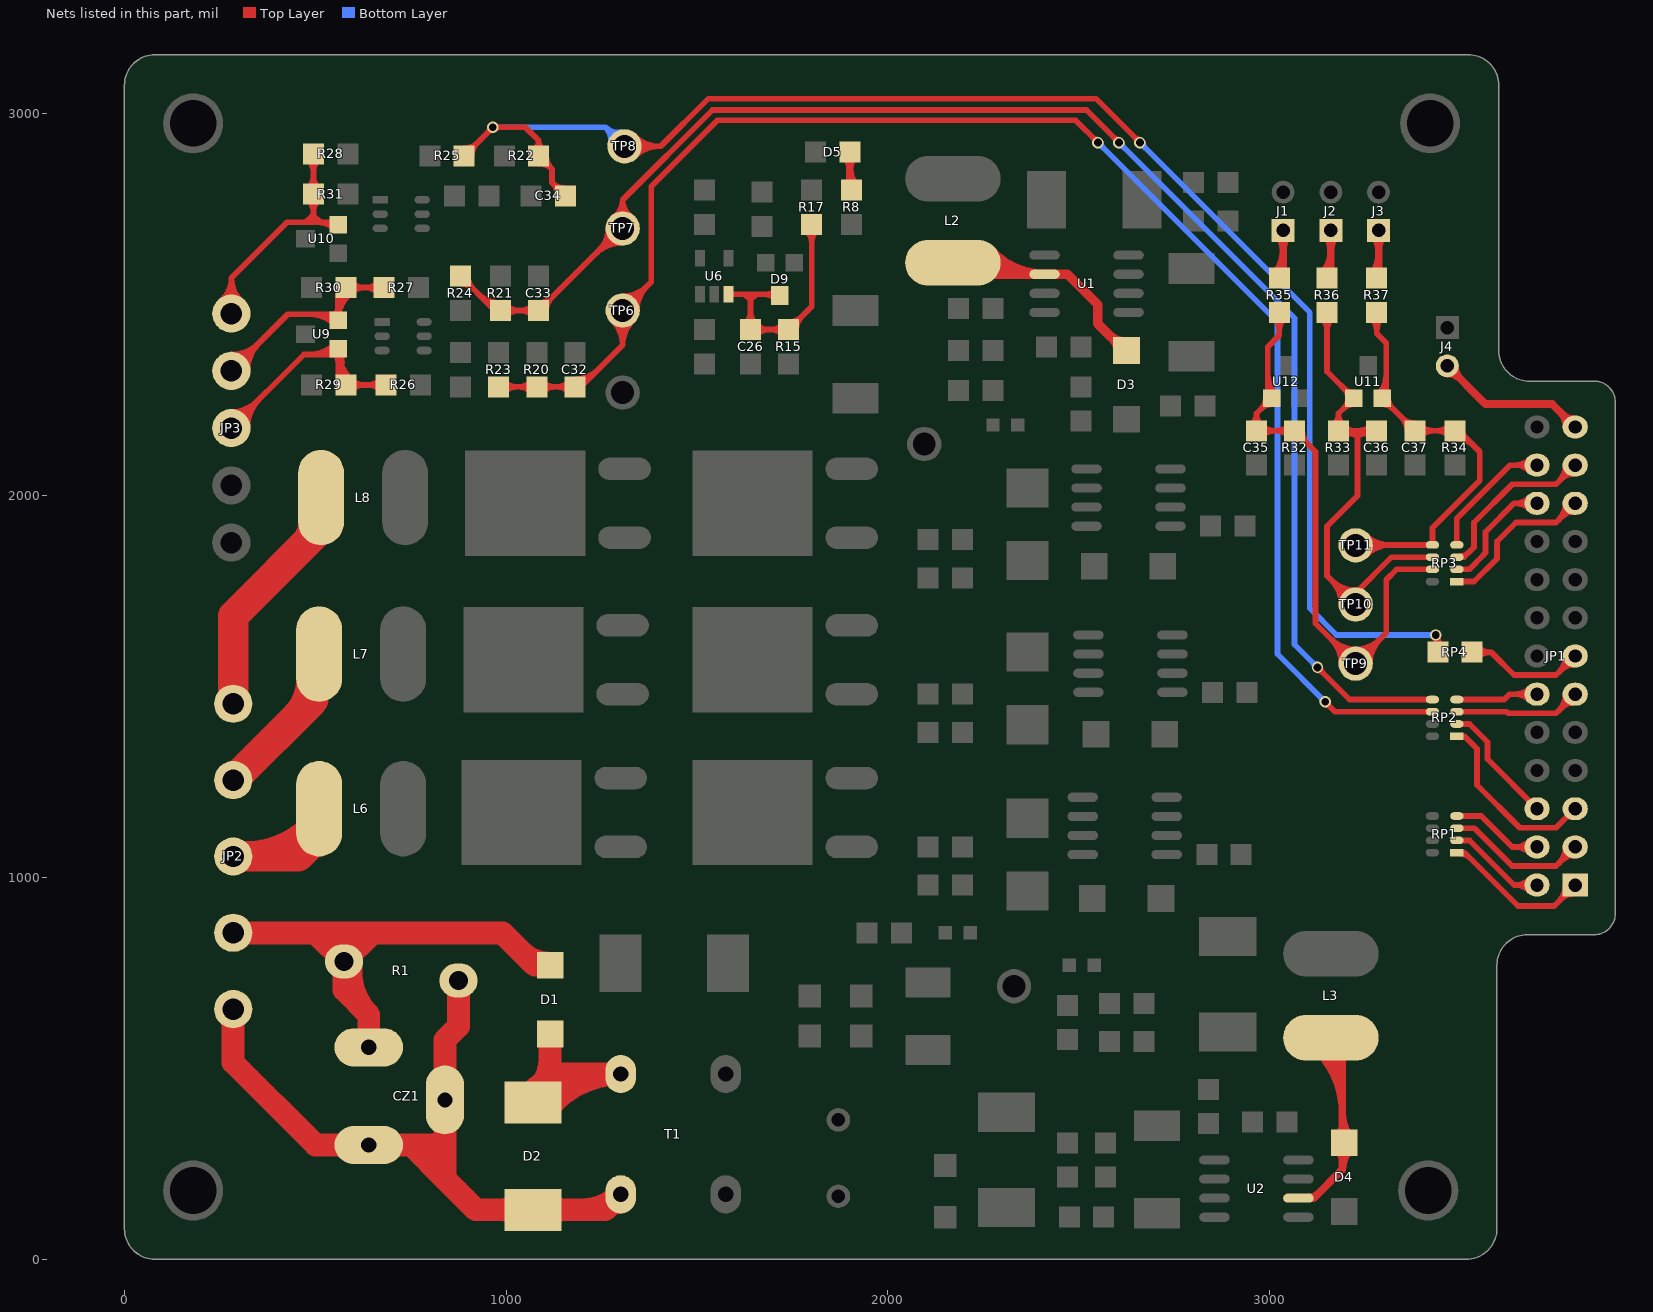
[diagram p0: the nets of this part, all layers, seen from the top]
# Altium PCB MISC103926.PcbDoc (part 3 of 4)
Units mil, origin at the board's own origin, x right, y up, seen from the top; angles counter-clockwise.
Board outline 3905 x 3155 mil, 4 copper layers (Top Layer, GND1, GND2, Bottom Layer); 132 components, 84 nets, 362 pads, 268 vias.

## Via types
v1: diameter 30, hole 20, Top Layer to Bottom Layer, 268 vias

## Nets (pads, with @x,y where several pads share a name; then routed paths per layer and width w, separated by ;. In a path a pad name is that pad's centre, name@x,y a point inside that pad or via, vN(x,y) a via of type N, cw(c..) or ccw(c..) an arc to the next point about the centre after c; other vN are vias at no path point) (continued)
NetC26_2: C26.2 D9.3 R15.1 R17.2 U6.3 | length 1114.7
  Top Layer w15: U6.3@1582.4,2527.76 1713.24,2527.76 D9.3@1717,2524 ; 1625,2527.76 1640,2512.76 ; C26.2@1625.86,2449.14 ccw(c1591.72,2483.28) 1640,2483.28 ccw(c1688.28,2483.28) 1654.14,2449.14 ccw(c1688.28,2483.28) 1688.28,2435 ccw(c1688.28,2386.72) C26.2@1654.14,2420.86 ; 1640,2527.76 1640,2510 ; 1655,2527.76 1640,2512.76 ; 1675.34,2527.76 cw(c1675.34,2484.34) D9.3@1706.04,2515.04 ; 1683.82,2527.76 ccw(c1683.82,2559.18) D9.3@1706.04,2536.96 ; R15.1@1725.86,2420.86 ccw(c1691.72,2386.72) 1691.72,2435 ccw(c1691.72,2483.28) R15.1@1725.86,2449.14 ; R15.1@1740,2455 ccw(c1740,2503.28) 1774.14,2469.14 ccw(c1808.28,2435) R15.1@1760,2435 ; R17.2@1785.86,2695.86 cw(c1751.72,2661.72) 1800,2661.72 cw(c1848.28,2661.72) R17.2@1814.14,2695.86 ; R17.2@1800,2710 1800,2495 R15.1@1740,2435 C26.2@1640,2435 1640,2510 ; 1640,2510 1640,2512.76 ; 1640,2510 1640,2512.76
NetC32_1: C32.1 R20.2 R23.1 RP2.6 TP6.1 | length 5058.5
  Top Layer w15: R23.1@985,2285 1195,2285 1305,2395 ; R23.1@994.14,2270.86 cw(c1028.28,2236.72) 1028.28,2285 cw(c1028.28,2333.28) R23.1@994.14,2299.14 ; R20.2@1065.86,2270.86 ccw(c1031.72,2236.72) 1031.72,2285 ccw(c1031.72,2333.28) R20.2@1065.86,2299.14 ; R20.2@1094.14,2270.86 cw(c1128.28,2236.72) 1128.28,2285 cw(c1128.28,2333.28) R20.2@1094.14,2299.14 ; C32.1@1165.86,2270.86 ccw(c1131.72,2236.72) 1131.72,2285 ccw(c1131.72,2333.28) C32.1@1165.86,2299.14 ; C32.1@1180,2290 ccw(c1180,2338.28) 1214.14,2304.14 ; C32.1@1180,2305 ccw(c1180,2389.5) 1239.75,2329.75 ; TP6.1@1278.6,2458.37 cw(c1215.76,2395.01) 1305,2395.01 ; TP6.1@1289.16,2469.02 cw(c1251.46,2431) 1305,2431 cw(c1358.54,2431) TP6.1@1320.84,2469.02 ; TP6.1@1305,2507.5 ccw(c1305,2561.82) 1343.41,2523.41 ccw(c1381.82,2485) TP6.1@1327.5,2485 ; TP6.1@1305,2522.5 ccw(c1305,2613.03) 1369.02,2549.02 ccw(c1433.03,2485) TP6.1@1342.5,2485 ; TP6.1@1331.4,2458.37 ccw(c1394.24,2395.01) 1305,2395.01 ; v1@2542.5,2925 ccw(c2524.39,2925) 2537.2,2937.8 ccw(c2550,2950.61) v1@2550,2932.5 ; v1(2550,2925) 2492,2983 1553,2983 1380,2810 1380,2560 TP6.1@1305,2485 1305,2395 ; v1@3145,1452.5 cw(c3145,1434.39) 3157.8,1447.2 cw(c3170.61,1460) v1@3152.5,1460 ; v1(3145,1460) 3171,1434 RP2.6@3426,1434
  Bottom Layer w15: v1@2550,2917.5 cw(c2550,2899.39) 2562.8,2912.2 cw(c2575.61,2925) v1@2557.5,2925 ; v1(2550,2925) 3020,2455 3020,1585 v1@3147.5,1457.5 ; v1@3137.5,1460 ccw(c3119.39,1460) 3132.2,1472.8 ccw(c3145,1485.61) v1@3145,1467.5
NetC33_1: C33.1 R21.2 R24.1 RP2.5 TP7.1 | length 4826.9
  Top Layer w15: R24.1@880,2555 cw(c880,2506.72) 914.14,2540.86 cw(c948.28,2575) R24.1@900,2575 ; R24.1@880,2575 R21.2@970,2485 ; 925.25,2529.75 ccw(c985,2589.5) R21.2@985,2505 ; 950.86,2504.14 ccw(c985,2538.28) R21.2@985,2490 ; R21.2@985,2485 C33.1@1090,2485 ; R21.2@999.14,2470.86 cw(c1033.28,2436.72) 1033.28,2485 cw(c1033.28,2533.28) R21.2@999.14,2499.14 ; C33.1@1070.86,2470.86 ccw(c1036.72,2436.72) 1036.72,2485 ccw(c1036.72,2533.28) C33.1@1070.86,2499.14 ; C33.1@1085,2485 TP7.1@1302.5,2702.5 ; C33.1@1085,2505 ccw(c1085,2553.28) 1119.14,2519.14 ccw(c1153.28,2485) C33.1@1105,2485 ; 1232.45,2632.45 cw(c1305,2559.9) TP7.1@1305,2662.5 ; 1244.52,2644.52 ccw(c1189.04,2700) TP7.1@1267.5,2700 ; 1258.05,2658.05 cw(c1305,2611.11) TP7.1@1305,2677.5 ; 1270.13,2670.13 ccw(c1240.25,2700) TP7.1@1282.5,2700 ; TP7.1@1282.5,2730 ccw(c1248.76,2775) 1305,2775 ; TP7.1@1305,2700 1305,2775 ; TP7.1@1327.5,2730 cw(c1361.24,2775) 1305,2775 ; v1@2597.5,2925 ccw(c2579.39,2925) 2592.2,2937.8 ccw(c2605,2950.61) v1@2605,2932.5 ; v1(2605,2925) 2520,3010 1540,3010 1305,2775 ; v1@3125,1542.5 cw(c3125,1524.39) 3137.8,1537.2 cw(c3150.61,1550) v1@3132.5,1550 ; v1(3125,1550) 3209,1466 RP2.5@3426,1466
  Bottom Layer w15: v1@2605,2917.5 cw(c2605,2899.39) 2617.8,2912.2 cw(c2630.61,2925) v1@2612.5,2925 ; v1(2605,2925) 3065,2465 3065,1610 v1(3125,1550) ; v1@3117.5,1550 ccw(c3099.39,1550) 3112.2,1562.8 ccw(c3125,1575.61) v1@3125,1557.5
NetC34_1: C34.1 R22.2 R25.1 RP4.2 TP8.1 | length 4924.8
  Top Layer w15: R25.1@890,2890 v1(965,2965) 1050,2965 1085,2930 ; R25.1@890,2910 ccw(c890,2958.28) 924.14,2924.14 ccw(c958.28,2890) R25.1@910,2890 ; v1@957.5,2965 cw(c939.4,2965) 952.2,2952.2 cw(c965,2939.4) v1@965,2957.5 ; v1@970.31,2959.7 cw(c983.1,2946.91) 983.1,2965 cw(c983.12,2983.12) v1@970.31,2970.31 ; R22.2@1073,2906 ccw(c1055,2930) 1085,2930 ; R22.2@1085,2870 cw(c1085,2821.72) 1119.14,2855.86 cw(c1153.28,2890) R22.2@1105,2890 ; R22.2@1097,2906 cw(c1115,2930) 1085,2930 ; C34.1@1135,2785 ccw(c1086.72,2785) 1120.86,2819.14 ccw(c1155,2853.28) C34.1@1155,2805 ; C34.1@1150,2790 1120,2820 1120,2855 R22.2@1085,2890 1085,2930 ; TP8.1@1310,2915 1405,2915 1530,3040 2545,3040 v1(2660,2925) ; TP8.1@1325.91,2899.09 cw(c1364.32,2860.68) 1364.32,2915 cw(c1364.32,2969.32) TP8.1@1325.91,2930.91 ; TP8.1@1336.52,2888.48 cw(c1400.53,2824.47) 1400.53,2915 cw(c1400.53,3005.53) TP8.1@1336.52,2941.52 ; v1@2652.5,2925 ccw(c2634.39,2925) 2647.2,2937.8 ccw(c2660,2950.61) v1@2660,2932.5 ; v1@2657.5,2922.5 v1@2657.5,2932.5 ; RP4.2@3428,1606 ccw(c3410,1630) v1@3440,1630 ; v1@3429.7,1629.7 cw(c3404.82,1604.82) RP4.2@3440,1604.82 ; v1@3431.25,1628.5 cw(c3416.16,1602.37) RP4.2@3445.31,1610.18 ; v1(3435,1635) v1@3440,1630 ; RP4.2@3440,1590 v1@3440,1630 ; RP4.2@3452,1606 cw(c3470,1630) v1@3440,1630
  Bottom Layer w15: v1(965,2965) 1260,2965 ; v1@970.31,2959.7 cw(c983.1,2946.91) 983.1,2965 cw(c983.12,2983.12) v1@970.31,2970.31 ; TP8.1@1273.17,2922.08 ccw(c1226.12,2931.12) 1260,2965 ; TP8.1@1302.92,2951.83 cw(c1293.88,2998.88) 1260,2965 ; TP8.1@1310,2915 1260,2965 ; v1@2660,2917.5 cw(c2660,2899.39) 2672.8,2912.2 cw(c2685.61,2925) v1@2667.5,2925 ; v1(2660,2925) 3105,2480 3105,1705 3175,1635 v1(3435,1635) ; v1@3429.7,1629.7 ccw(c3416.89,1616.89) 3416.89,1635 ccw(c3416.89,1653.11) v1@3429.7,1640.3
NetC35_2: C35.2 R32.1 R35.2 RP3.7 TP9.1 U12.1 | length 2488.9
  Top Layer w15: C35.2@2951.6,2184.85 ccw(c2924.38,2215) 2965,2215 ; C35.2@2978.4,2184.85 cw(c3005.62,2215) 2965,2215 ; C35.2@2979.14,2155.86 cw(c3013.28,2121.72) 3013.28,2170 cw(c3013.28,2218.28) C35.2@2979.14,2184.14 ; U12.1@2989.5,2255 cw(c2952.08,2255) 2978.54,2228.54 cw(c3005,2202.08) U12.1@3005,2239.5 ; 2995,2280.35 ccw(c3030.35,2280.35) U12.1@3005.35,2255.35 ; 2995,2316.56 ccw(c3066.56,2316.56) U12.1@3015.96,2265.96 ; R35.2@3010.86,2465.86 cw(c2976.72,2431.72) 3025,2431.72 cw(c3073.28,2431.72) R35.2@3039.14,2465.86 ; R35.2@3025,2470 R35.2@3025,2480 3025,2420 2995,2390 2995,2265 U12.1@3005,2255 2965,2215 ; R32.1@3050.86,2155.86 ccw(c3016.72,2121.72) 3016.72,2170 ccw(c3016.72,2218.28) R32.1@3050.86,2184.14 ; R32.1@3065,2150 cw(c3065,2101.72) 3099.14,2135.86 cw(c3133.28,2170) R32.1@3085,2170 ; R32.1@3065,2170 3120,2115 3120,1665 TP9.1@3225,1560 3305,1640 3305,1780 3332,1807 RP3.7@3426,1807 ; R32.1@3070,2170 C35.2@2965,2170 2965,2215 ; TP9.1@3187.5,1560 ccw(c3096.97,1560) 3160.98,1624.02 ccw(c3225,1688.03) 3225,1597.5 ccw(c3225,1688.03) 3289.02,1624.02 ccw(c3353.03,1560) TP9.1@3262.5,1560 ; TP9.1@3202.5,1560 ccw(c3148.18,1560) 3186.59,1598.41 ccw(c3225,1636.82) 3225,1582.5 ccw(c3225,1636.82) 3263.41,1598.41 ccw(c3301.82,1560) TP9.1@3247.5,1560
NetC36_2: C36.2 R33.1 R36.2 RP3.6 TP10.1 U11.1 | length 2143.9
  Top Layer w15: R36.2@3135.86,2465.86 cw(c3101.72,2431.72) 3150,2431.72 cw(c3198.28,2431.72) R36.2@3164.14,2465.86 ; R36.2@3150,2480 3150,2325 U11.1@3220,2255 3180,2215 ; R33.1@3166.6,2184.85 ccw(c3139.38,2215) 3180,2215 ; R33.1@3183.44,2166.37 cw(c3201.03,2147.82) 3219.11,2165.89 ; TP10.1@3187.5,1715 ccw(c3096.97,1715) 3160.98,1779.02 ccw(c3225,1843.03) TP10.1@3225,1752.5 ; R33.1@3193.4,2184.85 cw(c3220.62,2215) 3180,2215 ; R33.1@3193.76,2155.49 cw(c3211.63,2136.63) 3230,2155 ; R33.1@3196,2158 cw(c3220,2140) 3220,2170 ; R33.1@3196,2182 ccw(c3220,2200) 3220,2170 ; R33.1@3197.23,2159.85 cw(c3215,2149.38) 3215,2170 ; R33.1@3197.23,2180.15 ccw(c3215,2190.62) 3215,2170 ; R33.1@3198.46,2162.31 cw(c3210,2157.5) 3210,2170 ; R33.1@3198.46,2177.69 ccw(c3210,2182.5) 3210,2170 ; TP10.1@3202.5,1715 ccw(c3148.18,1715) 3186.59,1753.41 ccw(c3225,1791.82) TP10.1@3225,1737.5 ; U11.1@3220,2239.5 ccw(c3220,2202.08) 3193.54,2228.54 ccw(c3167.08,2255) 3204.5,2255 ccw(c3167.08,2255) 3193.54,2281.46 ccw(c3220,2307.92) U11.1@3220,2270.5 ; 3230,2170 3230,2155 ; 3240.89,2165.89 cw(c3258.97,2147.82) C36.2@3276.56,2166.37 ; 3245,2170 3230,2155 ; C36.2@3265.86,2155.86 ccw(c3231.72,2121.72) 3231.72,2170 ccw(c3231.72,2218.28) C36.2@3265.86,2184.14 ; C36.2@3266.24,2155.49 ccw(c3248.37,2136.63) 3230,2155 ; C36.2@3280,2170 3220,2170 ; RP3.6@3426,1839 3319,1839 3225,1745 TP10.1@3225,1715 3150,1790 3150,1920 3230,2000 3230,2155 ; 3180,2215 R33.1@3180,2170 3220,2170 ; 3210,2170 3215,2170 ; 3215,2170 3230,2155
NetC37_2: C37.2 R34.1 R37.2 RP3.5 TP11.1 U11.2 | length 1835.7
  Top Layer w15: TP11.1@3225,1870 3226,1871 RP3.5@3426,1871 3426,1916 3550,2040 3550,2115 3495,2170 R34.1@3485,2170 C37.2@3380,2170 U11.2@3295,2255 3305,2265 3305,2400 3280,2425 R37.2@3280,2480 R37.2@3286,2474 ; TP11.1@3240.91,1854.09 cw(c3281.74,1813.26) 3281.74,1871 ; TP11.1@3240.91,1885.91 ccw(c3276.9,1921.9) 3276.9,1871 ; TP11.1@3251.52,1843.48 cw(c3317.95,1777.05) 3317.95,1871 ; TP11.1@3251.52,1896.52 ccw(c3313.12,1958.12) 3313.12,1871 ; R37.2@3265.86,2465.86 cw(c3231.72,2431.72) 3280,2431.72 cw(c3328.28,2431.72) R37.2@3294.14,2465.86 ; U11.2@3284.04,2265.96 ccw(c3233.43,2316.56) 3305,2316.56 ; U11.2@3294.65,2255.35 ccw(c3269.65,2280.35) 3305,2280.35 ; U11.2@3295,2239.5 cw(c3295,2202.08) 3321.46,2228.54 cw(c3347.92,2255) U11.2@3310.5,2255 ; C37.2@3360,2170 ccw(c3311.72,2170) 3345.86,2204.14 ccw(c3380,2238.28) C37.2@3380,2190 ; C37.2@3394.14,2155.86 cw(c3428.28,2121.72) 3428.28,2170 cw(c3428.28,2218.28) C37.2@3394.14,2184.14 ; R34.1@3470.86,2155.86 ccw(c3436.72,2121.72) 3436.72,2170 ccw(c3436.72,2218.28) R34.1@3470.86,2184.14 ; R34.1@3485,2150 cw(c3485,2077.57) 3536.21,2128.79 ; R34.1@3485,2165 cw(c3485,2128.79) R34.1@3510.61,2154.39 ; R34.1@3505,2170 ccw(c3529.14,2170) R34.1@3512.07,2152.93
NetCZ1_1: CZ1.1 CZ1.3 D2.2 JP2.1 R1.2 T1.1 | length 2284.5
  Top Layer w60: JP2.1@284.55,654.55 284.55,515.45 500.91,299.09 833.46,299.09 839.37,305 ; 750.91,299.09 839.37,210.63 ; R1.2@875,730 875,610 839.37,574.37 CZ1.1@839.37,417.2 839.37,210.63 ; D2.2@1032.32,111.82 ccw(c989.64,69.14) 989.64,129.5 ccw(c989.64,189.86) D2.2@1032.32,147.18 ; D2.2@1107.68,111.82 cw(c1150.36,69.14) 1150.36,129.5 cw(c1150.36,189.86) D2.2@1107.68,147.18 ; 1202.22,129.5 ccw(c1202.22,257.78) T1.1@1292.93,167.07 ; 1265.86,135.86 cw(c1300,101.72) T1.1@1300,150 ; T1.1@1300,170 1259.5,129.5 D2.2@1070,129.5 920.5,129.5 839.37,210.63
NetCZ1_2: CZ1.2 D1.2 JP2.2 R1.1 | length 1572
  Top Layer w60: JP2.2@285,855 500,855 ; R1.1@570,775 R1.1@575,780 ; R1.1@594.83,777.73 ccw(c753.48,753.49) 640,640 ; CZ1.2@640,555 640,640 ; 1038.18,806.82 ccw(c1115,883.64) D1.2@1115,775 ; D1.2@1115,770 1075,770 990,855 650,855 ; 500,855 R1.1@575,780 ; 500,855 650,855 ; R1.1@575,780 575,705 640,640 ; R1.1@575,780 650,855
NetD1_1: D1.1 D2.1 T1.4 | length 841.9
  Top Layer w60: D2.1@1062.91,432.67 cw(c1173.36,342.28) 1173.36,485 ; D2.1@1070,410.5 1115,455.5 D1.1@1115,590 ; D2.1@1072.32,428.18 ccw(c969.29,531.21) 1115,531.21 ; D2.1@1109.35,394.67 cw(c1299.99,238.66) T1.4@1300,485 1115,485
NetD3_1: D3.1 L2.1 U1.2 | length 1009
  Top Layer w25: L2.1@2170,2610 2200,2580 U1.2@2410,2580 ; L2.1@2233.15,2608.32 ccw(c2297.09,2666.35) 2297.09,2580 ; L2.1@2251.66,2625.12 ccw(c2353.54,2717.58) 2353.54,2580 ; L2.1@2270.18,2641.92 ccw(c2409.99,2768.8) U1.2@2410,2580 ; 2578.05,2421.95 ccw(c2625,2468.89) D3.1@2625,2402.5 ; D3.1@2590.13,2409.87 cw(c2560.25,2380) D3.1@2602.5,2380 ; D3.1@2625,2380 2620,2380 2550,2450 2550,2500 2470,2580 U1.2@2410,2580
NetD4_1: D4.1 L3.1 U2.2 | length 1143.2
  Top Layer w20: U2.2@3075,160 3115,160 3190,235 3190,305 3190,550 L3.1@3160,580 L3.1@3150,570 ; U2.2@3103,162 ccw(c3103,195.8) 3126.9,171.9 ; L3.1@3124.65,544.64 cw(c2966.87,386.86) 3190,386.86 ; L3.1@3138.79,558.79 cw(c3015.15,435.15) 3190,435.15 ; L3.1@3152.93,572.93 cw(c3063.43,483.43) 3190,483.43 ; D4.1@3177.32,287.32 cw(c3146.72,256.72) 3190,256.72 ; D4.1@3177.32,322.68 ccw(c3146.72,353.28) 3190,353.28 ; 3190,234.83 cw(c3262.07,234.83) D4.1@3212.27,286.93 ; 3190,377.43 ccw(c3267.43,377.43) D4.1@3212.68,322.68
NetD5_1: D5.1 R8.2 | length 234.8
  Top Layer w20: D5.1@1887.63,2887.63 cw(c1857.75,2857.75) 1900,2857.75 cw(c1942.25,2857.75) D5.1@1912.37,2887.63 ; R8.2@1892.63,2812.37 ccw(c1874.82,2830.18) 1900,2830.18 ; 1900,2854.32 ccw(c1959.32,2854.32) R8.2@1917.37,2812.37 ; D5.1@1900,2900 1900,2805 R8.2@1905,2800
NetJ1_1: J1.1 R35.1 | length 265
  Top Layer w15: R35.1@3025,2570 R35.1@3035,2580
  Top Layer w20: R35.1@3012.63,2582.37 ccw(c2958.61,2636.39) 3035,2636.39 ; J1.1@3020.86,2680.86 cw(c2986.72,2646.72) 3035,2646.72 cw(c3083.29,2646.72) J1.1@3049.14,2680.86 ; R35.1@3035,2580 J1.1@3035,2695
NetJ2_1: J2.1 R36.1 | length 265
  Top Layer w15: R36.1@3150,2570 R36.1@3160,2580
  Top Layer w20: R36.1@3137.63,2582.37 ccw(c3083.61,2636.39) 3160,2636.39 ; J2.1@3145.86,2680.86 cw(c3111.72,2646.72) 3160,2646.72 cw(c3208.29,2646.72) J2.1@3174.14,2680.86 ; R36.1@3160,2580 J2.1@3160,2695
NetJ3_1: J3.1 R37.1 | length 269.3
  Top Layer w15: R37.1@3280,2570 R37.1@3285,2575
  Top Layer w20: R37.1@3267.63,2582.37 ccw(c3225.68,2624.32) 3285,2624.32 ; J3.1@3270.86,2680.86 cw(c3236.72,2646.72) 3285,2646.72 cw(c3333.29,2646.72) J3.1@3299.14,2680.86 ; R37.1@3285,2575 J3.1@3285,2695 ; 3285,2600.18 ccw(c3310.18,2600.18) R37.1@3292.37,2582.37
NetJ4_2: J4.2 JP1.25 | length 553
  Top Layer w20: J4.2@3465,2320 cw(c3465,2271.72) 3499.14,2305.86 cw(c3533.28,2340) J4.2@3485,2340 ; J4.2@3465,2340 3565,2240 3740,2240 JP1.25@3800,2180 ; 3760.74,2219.26 cw(c3721.47,2180) JP1.25@3777,2180 ; 3767.98,2212.02 ccw(c3797,2241.04) JP1.25@3797,2200
NetJP1_1: JP1.1 RP1.1 | length 504.5
  Top Layer w15: RP1.1@3490,1065 3510,1065 3650,925 3745,925 JP1.1@3800,980 ; RP1.1@3497.5,1062.5 cw(c3497.5,1026.29) 3523.11,1051.89 ; 3756.47,936.47 ccw(c3712.94,980) JP1.1@3774.5,980 ; 3763.71,943.71 cw(c3797,910.42) JP1.1@3797,957.5
NetJP1_2: JP1.2 RP1.2 | length 343.8
  Top Layer w15: RP1.2@3490,1097 3523,1097 3640,980 JP1.2@3700,980 ; JP1.2@3681.09,964.09 ccw(c3642.68,925.68) 3642.68,980 ccw(c3642.68,1034.32) JP1.2@3681.09,995.91
NetJP1_3: JP1.3 RP1.3 | length 457
  Top Layer w15: RP1.3@3490,1129 3536,1129 3635,1030 3750,1030 JP1.3@3800,1080 ; 3756.47,1036.47 ccw(c3712.94,1080) JP1.3@3774.5,1080 ; 3763.71,1043.71 cw(c3797,1010.42) JP1.3@3797,1057.5
NetJP1_4: JP1.4 RP1.4 | length 328.9
  Top Layer w15: RP1.4@3490,1161 3554,1161 3635,1080 JP1.4@3700,1080 ; JP1.4@3681.09,1064.09 ccw(c3642.68,1025.68) 3642.68,1080 ccw(c3642.68,1134.32) JP1.4@3681.09,1095.91
NetJP1_5: JP1.5 RP2.1 | length 485.8
  Top Layer w15: RP2.1@3490,1370 3510,1370 3543,1337 3543,1242 3655,1130 3750,1130 JP1.5@3800,1180
NetJP1_6: JP1.6 RP2.2 | length 328.3
  Top Layer w15: RP2.2@3490,1402 3523,1402 3570,1355 3570,1310 JP1.6@3700,1180
NetJP1_11: JP1.11 RP2.3 | length 417.7
  Top Layer w15: RP2.3@3490,1434 3620,1434 3624,1430 3750,1430 JP1.11@3800,1480 ; 3756.47,1436.47 ccw(c3712.94,1480) JP1.11@3774.5,1480 ; 3763.71,1443.71 cw(c3797,1410.42) JP1.11@3797,1457.5
NetJP1_12: JP1.12 RP2.4 | length 301.1
  Top Layer w15: RP2.4@3490,1466 3614,1466 3628,1480 JP1.12@3700,1480 ; JP1.12@3681.09,1464.09 ccw(c3642.68,1425.68) 3642.68,1480 ccw(c3642.68,1534.32) JP1.12@3681.09,1495.91
NetJP1_13: JP1.13 RP4.1 | length 476.7
  Top Layer w15: RP4.1@3530,1590 3580,1590 3640,1530 3750,1530 JP1.13@3800,1580 ; RP4.1@3544.14,1575.86 cw(c3578.28,1541.72) 3578.28,1590 cw(c3578.28,1638.28) RP4.1@3544.14,1604.14 ; 3756.47,1536.47 ccw(c3712.94,1580) JP1.13@3774.5,1580 ; 3763.71,1543.71 cw(c3797,1510.42) JP1.13@3797,1557.5
NetJP1_21: JP1.21 RP3.1 | length 506.6
  Top Layer w15: RP3.1@3490,1775 3535,1775 3595,1835 3595,1880 3645,1930 3750,1930 JP1.21@3800,1980 ; 3756.47,1936.47 ccw(c3712.94,1980) JP1.21@3774.5,1980 ; 3763.71,1943.71 cw(c3797,1910.42) JP1.21@3797,1957.5
NetJP1_22: JP1.22 RP3.2 | length 399.4
  Top Layer w15: RP3.2@3490,1807 3522.36,1807 3560,1844.64 3560,1845 3565.18,1850.18 3565.18,1905.18 3640,1980 JP1.22@3700,1980 ; JP1.22@3681.09,1964.09 ccw(c3642.68,1925.68) 3642.68,1980 ccw(c3642.68,2034.32) JP1.22@3681.09,1995.91
NetJP1_23: JP1.23 RP3.3 | length 559.8
  Top Layer w15: RP3.3@3490,1839 3509,1839 3535,1865 3535,1930 3635,2030 3750,2030 JP1.23@3800,2080 ; RP3.3@3497.5,1841.5 ccw(c3497.5,1875.3) 3521.4,1851.4 ; 3756.47,2036.47 ccw(c3712.94,2080) JP1.23@3774.5,2080 ; 3763.71,2043.71 cw(c3797,2010.42) JP1.23@3797,2057.5
NetJP1_24: JP1.24 RP3.4 | length 422.3
  Top Layer w15: RP3.4@3490,1871 3490,1940 3630,2080 JP1.24@3700,2080 ; JP1.24@3681.09,2064.09 ccw(c3642.68,2025.68) 3642.68,2080 ccw(c3642.68,2134.32) JP1.24@3681.09,2095.91
NetJP2_3: JP2.3 L6.2 | length 510.4
  Top Layer w60: L6.2@495,1095 L6.2@495,1180
  Top Layer w80: JP2.3@285,1055 455,1055 L6.2@495,1095 ; JP2.3@316.86,1055 ccw(c316.86,1308.14) L6.2@495.86,1129.14
NetJP2_4: JP2.4 L7.2 | length 566.1
  Top Layer w60: L7.2@485,1585 L7.2@510,1560
  Top Layer w80: JP2.4@285,1255 495,1465 L7.2@495,1585 ; 447.57,1417.57 ccw(c345.14,1520) L7.2@490,1520
NetJP2_5: JP2.5 L8.2 | length 701.6
  Top Layer w80: JP2.5@285,1455 285,1685 515,1915 L8.2@515,1995 ; 470.25,1870.25 ccw(c410.5,1930) L8.2@495,1930
NetJP3_3: JP3.3 R26.2 R29.1 U9.1 | length 1401.1
  Top Layer w15: JP3.3@278.5,2178.5 470,2370 U9.1@560,2370 ; JP3.3@280,2204.5 ccw(c280,2263.65) 321.82,2221.82 ; JP3.3@280,2219.5 ccw(c280,2314.86) 347.43,2247.43 ; JP3.3@307.5,2177 cw(c381.13,2177) 329.07,2229.07 ; JP3.3@322.5,2177 cw(c432.35,2177) 354.67,2254.67 ; 486.37,2370 ccw(c486.37,2458.63) U9.1@549.04,2395.96 ; 522.58,2370 ccw(c522.58,2422.42) U9.1@559.65,2385.35 ; U9.1@549.04,2374.04 cw(c522.58,2347.58) 560,2347.58 cw(c597.42,2347.58) U9.1@570.96,2374.04 ; U9.1@552.25,2371.58 cw(c533.54,2339.17) 569.68,2348.86 cw(c605.83,2358.54) U9.1@573.42,2377.25 ; R29.1@560,2313.75 ccw(c603.2,2313.75) R29.1@573.01,2282.85 ; 560,2349.37 ccw(c638,2349.37) R29.1@583.49,2293.58 ; R29.1@593.98,2304.31 cw(c672.8,2384.99) U9.1@560,2385 560,2310 R29.1@580,2290 R26.2@685,2290 ; R29.1@594.14,2275.86 cw(c628.28,2241.72) 628.28,2290 cw(c628.28,2338.28) R29.1@594.14,2304.14 ; R26.2@670.86,2275.86 ccw(c636.72,2241.72) 636.72,2290 ccw(c636.72,2338.28) R26.2@670.86,2304.14
NetJP3_4: JP3.4 R27.2 R30.1 U9.2 | length 1296.2
  Top Layer w15: JP3.4@280,2327 428,2475 U9.2@559,2475 ; JP3.4@280,2354.5 ccw(c280,2420.89) 326.95,2373.95 ccw(c373.89,2327) JP3.4@307.5,2327 ; JP3.4@280,2369.5 ccw(c280,2472.1) 352.55,2399.55 ccw(c425.1,2327) JP3.4@322.5,2327 ; 486.36,2475 cw(c486.36,2386.36) U9.2@549.04,2449.04 ; 522.58,2475 cw(c522.58,2422.58) U9.2@559.65,2459.65 ; U9.2@549.04,2470.96 ccw(c524.99,2495.01) 559,2495.01 ; U9.2@559,2458.42 cw(c650.92,2458.42) R30.1@592.67,2529.53 ; 559,2490.09 cw(c624.97,2490.09) R30.1@583.17,2541.13 ; 559,2499.83 ccw(c599.83,2499.83) U9.2@570.96,2470.96 ; R30.1@559,2521.77 cw(c599.03,2521.77) R30.1@573.66,2552.74 ; U9.2@560,2460 559,2461 559,2524 R30.1@580,2545 R27.2@680,2545 ; R30.1@594.14,2530.86 cw(c628.28,2496.72) 628.28,2545 cw(c628.28,2593.28) R30.1@594.14,2559.14 ; R27.2@665.86,2530.86 ccw(c631.72,2496.72) 631.72,2545 ccw(c631.72,2593.28) R27.2@665.86,2559.14
NetJP3_5: JP3.5 R28.2 R31.1 U10.2 | length 1185.3
  Top Layer w15: JP3.5@252.19,2509.13 ccw(c199.51,2570) 280,2570 ; JP3.5@262,2497.79 ccw(c227.92,2537.17) 280,2537.17 ccw(c332.08,2537.17) JP3.5@298,2497.79 ; JP3.5@280,2477 280,2570 ; JP3.5@307.81,2509.13 cw(c360.49,2570) 280,2570 ; 475,2716 494,2735 ; R31.1@480.86,2775.86 cw(c446.72,2741.72) 495,2741.72 cw(c543.28,2741.72) R31.1@509.14,2775.86 ; R31.1@480.86,2804.14 ccw(c446.72,2838.28) 495,2838.28 ccw(c543.28,2838.28) R31.1@509.14,2804.14 ; R28.2@480.86,2880.86 cw(c446.72,2846.72) 495,2846.72 cw(c543.28,2846.72) R28.2@509.14,2880.86 ; 495,2716 495,2735 ; R28.2@495,2895 R31.1@495,2790 495,2735 ; 508.09,2716 cw(c508.09,2658.09) U10.2@549.04,2699.04 ; 515,2716 513,2716 494,2735 ; U10.2@537.07,2716 ccw(c537.07,2732.93) U10.2@549.04,2720.96 ; U10.2@554,2716 426,2716 280,2570 ; 494,2735 495,2735
  Top Layer w20: U10.2@554,2716 U10.2@560,2710